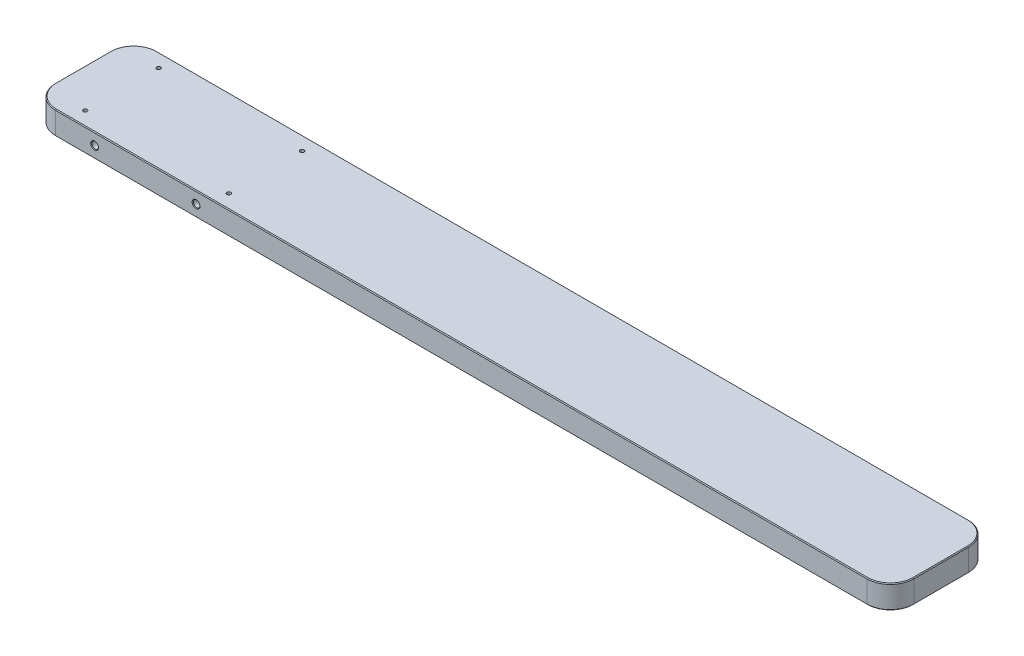
SolidWorks part; units mm, degrees
ref_plane "Front Plane" through (0, 0, 0) normal (0, 0, 1) x (1, 0, 0)
ref_plane "Top Plane" through (0, 0, 0) normal (0, 1, 0) x (1, 0, 0)
ref_plane "Right Plane" through (0, 0, 0) normal (1, 0, 0) x (0, 0, -1)
sketch "Sketch1" plane through (0, 0, 0) normal (0, 1, 0) x (1, 0, 0)
  line L1 (-550, -65) -> (550, -65)
  line L2 (-550, -65) -> (-550, 65)
  line L3 (-550, 65) -> (550, 65)
  line L4 (550, -65) -> (550, 65)
  line L5 (-550, -65) -> (550, 65) construction
  line L6 (-550, 65) -> (550, -65) construction
  point P1 (0, 0)
  dimension "D1" = 1100
  dimension "D2" = 130
extrude "Boss-Extrude1" add sketch "Sketch1" along normal blind 30
sketch "Sketch4" plane through (0, 30, 0) normal (0, 1, 0) x (1, 0, 0)
  line L0 (-550, 65) -> (-550, -65) construction
  line L1 (-500, -47) -> (-316, -47) construction
  line L2 (-500, -47) -> (-500, 47) construction
  line L3 (-500, 47) -> (-316, 47) construction
  line L4 (-316, -47) -> (-316, 47) construction
  line L5 (-500, -47) -> (-316, 47) construction
  line L6 (-500, 47) -> (-316, -47) construction
  point P0 (-408, 0)
  dimension "D1" = 184
  dimension "D2" = 94
  dimension "D3" = 50
hole_wizard "M6 Tapped Hole1" positions "Sketch5" profile "Sketch6" tap size "M6" standard "GB" end condition through all
sketch "Sketch5" plane through (0, 30, 0) normal (0, 1, 0) x (1, 0, 0)
  point P0 (-316, 47)
  point P3 (-316, -47)
  point P6 (-500, 47)
  point P9 (-500, -47)
cosmetic thread "Cosmetic thread 1" parameters "D2"=6
cosmetic thread "Cosmetic thread 2" parameters "D2"=6
cosmetic thread "Cosmetic thread 3" parameters "D2"=6
cosmetic thread "Cosmetic thread 4" parameters "D2"=6
sketch "Sketch6" plane through (-316, 30, -47) normal (1, 0, 0) x (0, 0, 1)
  line L0 (0, 0) -> (0, 30)
  line L1 (0, 30) -> (2.5, 30)
  line L2 (2.5, 30) -> (2.5, 0)
  line L5 (2.5, 0) -> (0, 0)
  line L11 (0, -6.35) -> (0, 107.95) construction
  dimension "通孔螺纹孔钻头直径" = 5
  dimension "通孔螺纹孔钻头深度" = 30
hole_wizard "M12 Tapped Hole1" positions "Sketch7" profile "Sketch9" tap size "M12" standard "GB"
sketch "Sketch7" plane through (0, 0, 0) normal (0, -1, 0) x (-1, 0, 0)
  line L0 (-1000, 0) -> (49000, 0) construction
  line L1 (550, 65) -> (550, -65) construction
  line L2 (-550, -65) -> (-550, 65) construction
  point P6 (-450, 0)
  point P8 (450, 0)
  dimension "D1" = 100
  dimension "D2" = 100
sketch "Sketch9" plane through (-450, 0, 0) normal (1, 0, 0) x (0, 0, -1)
  line L0 (0, 0) -> (0, 28.0644)
  line L1 (0, 28.0644) -> (5.1, 25)
  line L2 (5.1, 25) -> (5.1, 0)
  line L5 (5.1, 0) -> (0, 0)
  line L10 (0, 28.0644) -> (-5.1, 25) construction
  line L11 (0, -6.35) -> (0, 107.95) construction
  dimension "螺纹孔钻头直径" = 10.2
  dimension "螺纹孔钻头深度" = 25
  dimension "导头角度" = 118
cosmetic thread "Cosmetic thread 5" parameters "D1"=24, "D2"=12
cosmetic thread "Cosmetic thread 6" parameters "D1"=24, "D2"=12
fillet "Fillet1" radius 30 4 edges at (550, 15, -65) (550, 15, 65) (-550, 15, 65) (-550, 15, -65)
chamfer "Chamfer1" distance 1 angle 45 16 edges at (-550, 0, 0) (0, 30, -65) (-541.2132, 0, 56.2132) (541.2132, 30, -56.2132) (0, 0, 65) (550, 30, 0) (541.2132, 0, 56.2132) (541.2132, 30, 56.2132) (550, 0, 0) (0, 30, 65) (541.2132, 0, -56.2132) (-541.2132, 30, 56.2132) (0, 0, -65) (-550, 30, 0) (-541.2132, 0, -56.2132) (-541.2132, 30, -56.2132)
hole_wizard "M10 Tapped Hole1" positions "Sketch10" profile "Sketch12" tap size "M10" standard "GB" end condition through all
sketch "Sketch10" plane through (0, 0, 65) normal (0, 0, 1) x (1, 0, 0)
  line L0 (520, 0) -> (-520, 0) construction
  line L2 (-550, 1) -> (-550, 29) construction
  point P0 (-470, 15)
  point P2 (-340, 15)
  dimension "D1" = 15
  dimension "D2" = 15
  dimension "D3" = 80
  dimension "D4" = 130
sketch "Sketch12" plane through (-470, 15, 65) normal (1, 0, 0) x (0, -1, 0)
  line L0 (0, 0) -> (0, 130)
  line L1 (0, 130) -> (4.25, 130)
  line L2 (4.25, 130) -> (4.25, 0.775)
  line L3 (4.25, 0.775) -> (5.025, 0)
  line L5 (5.025, 0) -> (0, 0)
  line L6 (-4.25, 0.775) -> (-5.025, 0) construction
  line L11 (0, -6.35) -> (0, 107.95) construction
  dimension "通孔螺纹孔钻头直径" = 8.5
  dimension "通孔螺纹孔钻头深度" = 130
  dimension "近端锥形沉头孔直径" = 10.05
  dimension "近端锥形沉头孔角度" = 90
cosmetic thread "Cosmetic thread 7" parameters "D2"=10
cosmetic thread "Cosmetic thread 8" parameters "D2"=10
